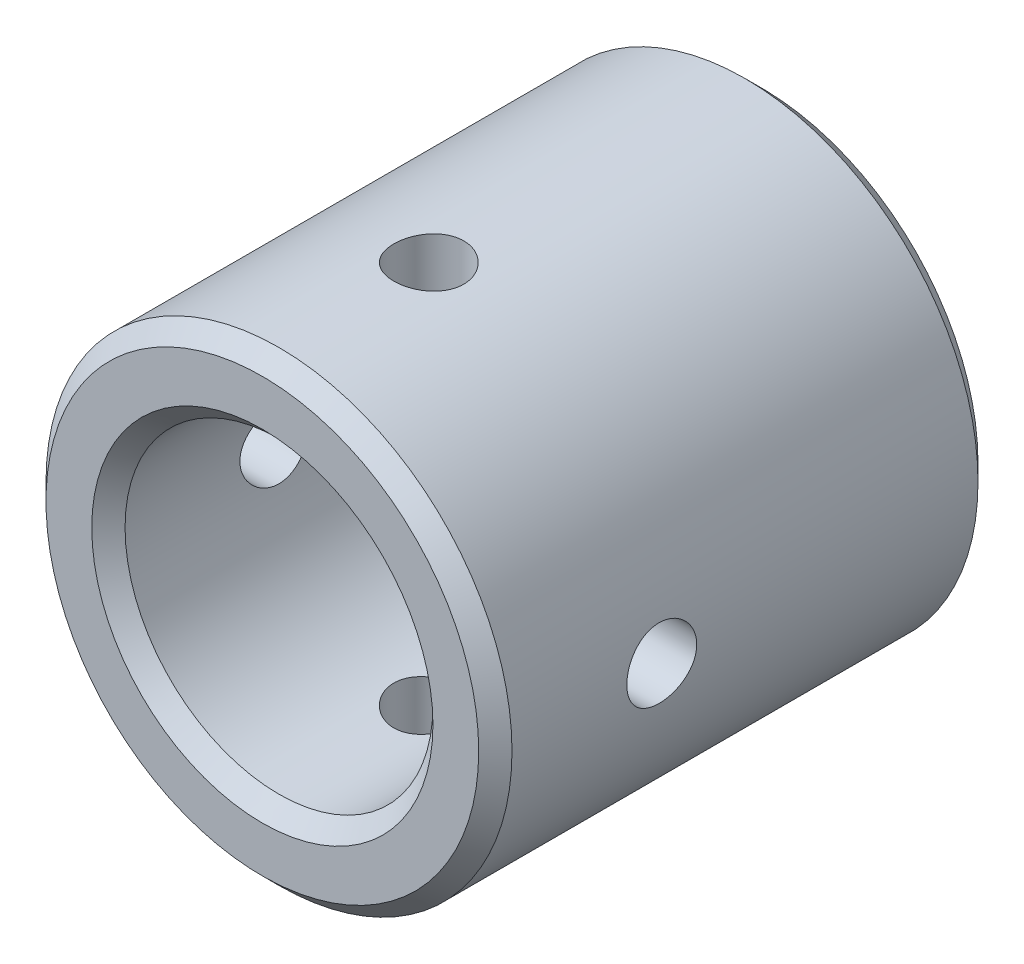
SolidWorks part; units mm, degrees
material "黑赛钢"
ref_plane "Front Plane" through (0, 0, 0) normal (0, 0, 1) x (1, 0, 0)
ref_plane "Top Plane" through (0, 0, 0) normal (0, 1, 0) x (1, 0, 0)
ref_plane "Right Plane" through (0, 0, 0) normal (1, 0, 0) x (0, 0, -1)
sketch "Sketch1" plane through (0, 0, 0) normal (0, 0, 1) x (1, 0, 0)
  circle A0 centre (0, 0) radius 14
  circle A1 centre (0, 0) radius 9.25
  dimension "D1" = 28
  dimension "D2" = 18.5
extrude "Boss-Extrude1" add sketch "Sketch1" along normal mid plane 30
hole_wizard "M5 Tapped Hole1" positions "Sketch3" profile "Sketch2" tap size "M5" standard "GB"
sketch "Sketch3" plane through (0, 0, 0) normal (0, 1, 0) x (1, 0, 0)
  point P0 (0, -5)
  dimension "D1" = 5
sketch "Sketch2" plane through (0, 0, 5) normal (1, 0, 0) x (0, 0, 1)
  line L0 (0, 0) -> (0, 14)
  line L1 (0, 14) -> (2.1, 14)
  line L2 (2.1, 14) -> (2.1, 0)
  line L5 (2.1, 0) -> (0, 0)
  line L11 (0, -6.35) -> (0, 107.95) construction
  dimension "通孔螺纹孔钻头直径" = 4.2
  dimension "通孔螺纹孔钻头深度" = 14
cosmetic thread "Hole Thread1" parameters "D2"=5
hole_wizard "M5 Tapped Hole2" positions "Sketch5" profile "Sketch4" tap size "M5" standard "GB"
sketch "Sketch5" plane through (0, 0, 0) normal (1, 0, 0) x (0, -1, 0)
  point P0 (0, -5)
  dimension "D1" = 5
sketch "Sketch4" plane through (0, 0, 5) normal (0, 1, 0) x (0, 0, 1)
  line L0 (0, 0) -> (0, 14)
  line L1 (0, 14) -> (2.1, 14)
  line L2 (2.1, 14) -> (2.1, 0)
  line L5 (2.1, 0) -> (0, 0)
  line L11 (0, -6.35) -> (0, 107.95) construction
  dimension "通孔螺纹孔钻头直径" = 4.2
  dimension "通孔螺纹孔钻头深度" = 14
cosmetic thread "Hole Thread2" parameters "D2"=5
hole_wizard "M5 Tapped Hole3" positions "Sketch9" profile "Sketch8" tap size "M5" standard "GB" end condition through all
sketch "Sketch9" plane through (0, 0, 0) normal (0, 1, 0) x (1, 0, 0)
  circle A0 centre (0, -5) radius 2.1 construction
  point P0 (0, -5)
sketch "Sketch8" plane through (0, 0, 5) normal (1, 0, 0) x (0, 0, -1)
  line L0 (0, 0) -> (0, 14)
  line L1 (0, 14) -> (2.1, 14)
  line L2 (2.1, 14) -> (2.1, 0)
  line L5 (2.1, 0) -> (0, 0)
  line L11 (0, -6.35) -> (0, 107.95) construction
  dimension "通孔螺纹孔钻头直径" = 4.2
  dimension "通孔螺纹孔钻头深度" = 14
cosmetic thread "Hole Thread7" parameters "D2"=5
hole_wizard "M5 Tapped Hole4" positions "Sketch11" profile "Sketch10" tap size "M5" standard "GB" end condition through all
sketch "Sketch11" plane through (0, 0, 0) normal (1, 0, 0) x (0, 0, -1)
  point P0 (-5, 0)
sketch "Sketch10" plane through (0, 0, 5) normal (0, 1, 0) x (0, 0, -1)
  line L0 (0, 0) -> (0, 14)
  line L1 (0, 14) -> (2.1, 14)
  line L2 (2.1, 14) -> (2.1, 0)
  line L5 (2.1, 0) -> (0, 0)
  line L11 (0, -6.35) -> (0, 107.95) construction
  dimension "通孔螺纹孔钻头直径" = 4.2
  dimension "通孔螺纹孔钻头深度" = 14
cosmetic thread "Hole Thread8" parameters "D2"=5
hole_wizard "M3 Tapped Hole1" positions "Sketch7" profile "Sketch6" tap size "M3" standard "GB"
sketch "Sketch7" plane through (0, 0, -15) normal (0, 0, -1) x (-1, 0, 0)
  line L1 (-6, -10) -> (6, -10) construction
  line L2 (-6, -10) -> (-6, 10) construction
  line L3 (-6, 10) -> (6, 10) construction
  line L4 (6, -10) -> (6, 10) construction
  line L5 (-6, -10) -> (6, 10) construction
  line L6 (-6, 10) -> (6, -10) construction
  point P0 (6, 10)
  point P2 (6, -10)
  point P4 (-6, -10)
  point P6 (-6, 10)
  dimension "D1" = 20
  dimension "D2" = 12
cosmetic thread "Hole Thread3" parameters "D1"=6, "D2"=3
cosmetic thread "Hole Thread4" parameters "D1"=6, "D2"=3
cosmetic thread "Hole Thread5" parameters "D1"=6, "D2"=3
cosmetic thread "Hole Thread6" parameters "D1"=6, "D2"=3
sketch "Sketch6" plane through (-6, 10, -15) normal (1, 0, 0) x (0, 1, 0)
  line L0 (0, 0) -> (0, 8.2511)
  line L1 (0, 8.2511) -> (1.25, 7.5)
  line L2 (1.25, 7.5) -> (1.25, 0)
  line L5 (1.25, 0) -> (0, 0)
  line L10 (0, 8.2511) -> (-1.25, 7.5) construction
  line L11 (0, -6.35) -> (0, 107.95) construction
  dimension "螺纹孔钻头直径" = 2.5
  dimension "螺纹孔钻头深度" = 7.5
  dimension "导头角度" = 118
chamfer "Chamfer1" distance 1 angle 45 4 edges at (9.25, 0, -15) (14, 0, -15) (9.25, 0, 15) (14, 0, 15)
